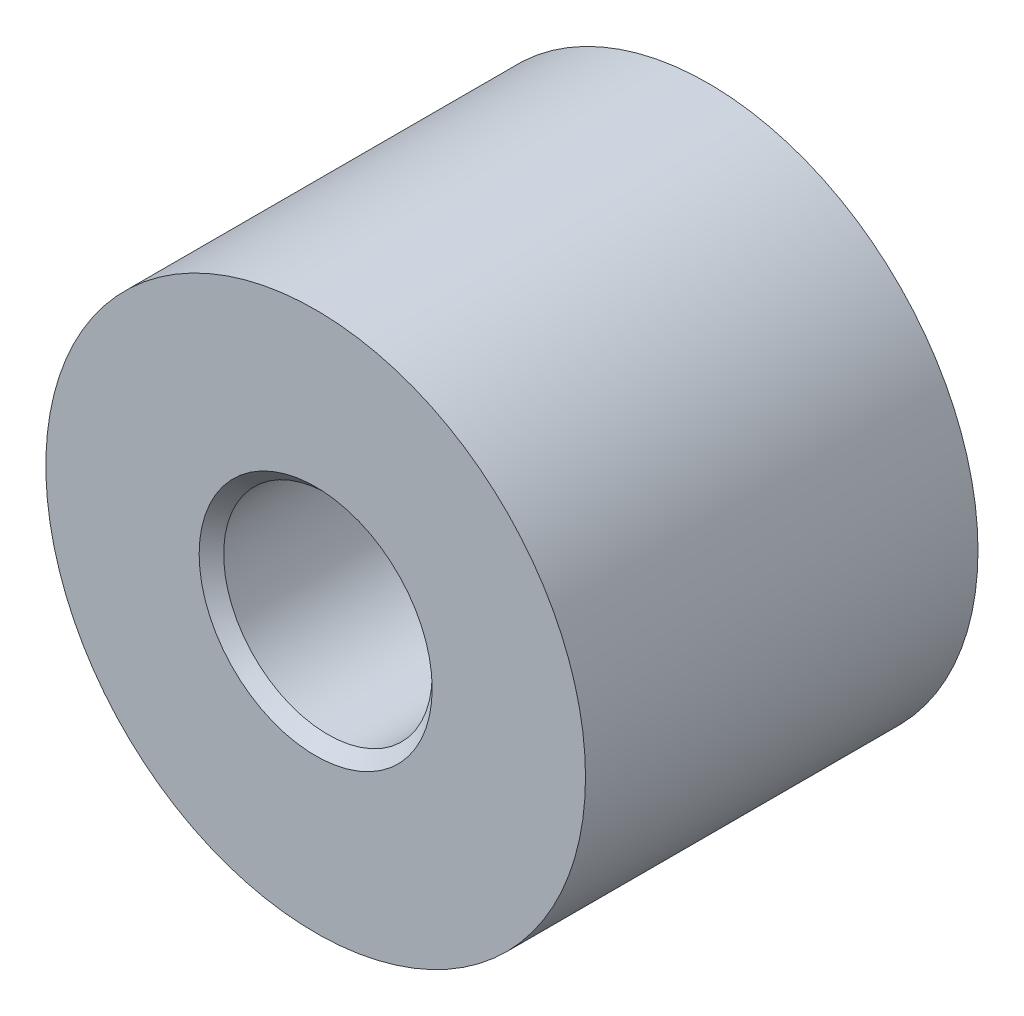
from build123d import *

# Parameters (mm, degrees)
SKETCH1_R           = 11
BOSS_EXTRUDE1_DEPTH = 16
SKETCH2_R           = 4.25
CUT_EXTRUDE1_DEPTH  = 16
CHAMFER1_SIZE       = 0.5


with BuildPart() as part:
    # Sketch1 → Boss-Extrude1 (new body)
    with BuildSketch(Plane.XY):
        Circle(SKETCH1_R)
    extrude(amount=BOSS_EXTRUDE1_DEPTH)

    # Sketch2 → Cut-Extrude1 (cut)
    with BuildSketch(Plane.XY.offset(16)):
        Circle(SKETCH2_R)
    extrude(amount=-CUT_EXTRUDE1_DEPTH, mode=Mode.SUBTRACT)

    # Chamfer1
    chamfer1_edges = [part.edges().sort_by_distance(p)[0] for p in [
        (-4.25, 0, 0),
        (-4.25, 0, 16),
    ]]
    chamfer(chamfer1_edges, length=CHAMFER1_SIZE)


solid = part.part
